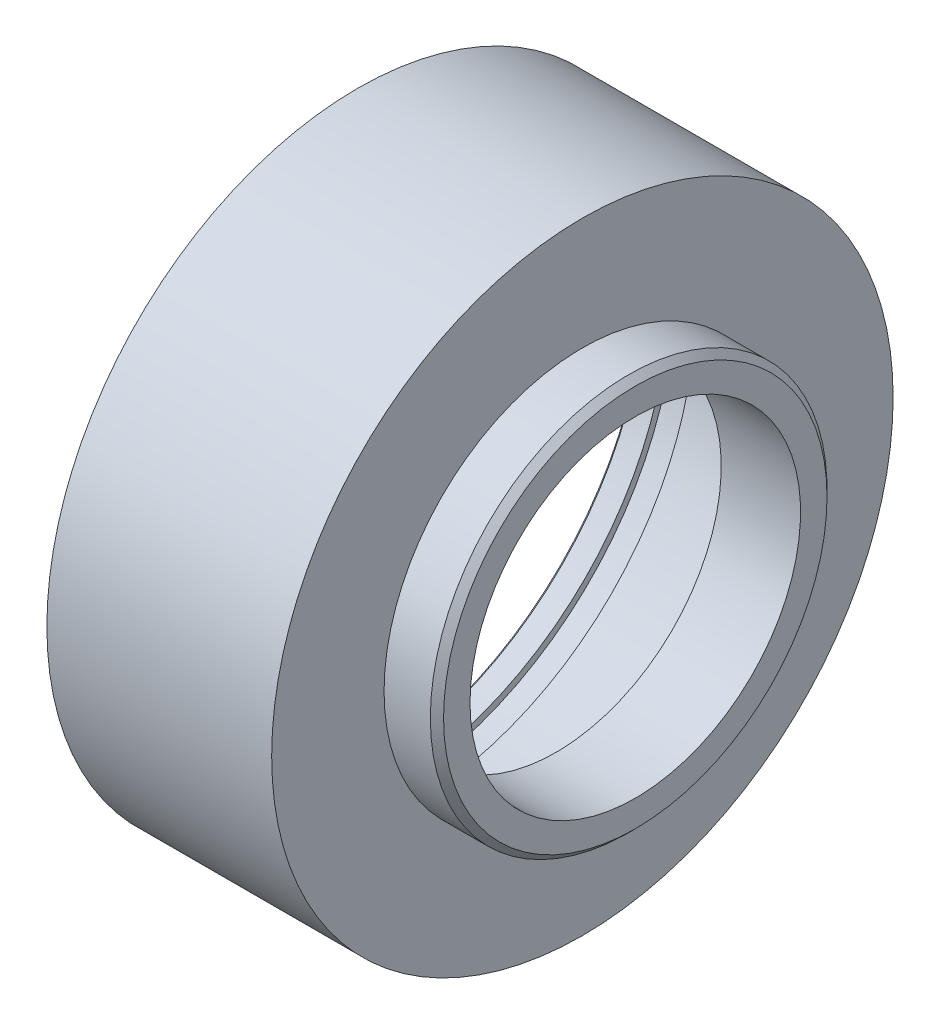
SolidWorks part; units mm, degrees
ref_plane "前视基准面" through (0, 0, 0) normal (0, 0, 1) x (1, 0, 0)
ref_plane "上视基准面" through (0, 0, 0) normal (0, 1, 0) x (1, 0, 0)
ref_plane "右视基准面" through (0, 0, 0) normal (1, 0, 0) x (0, 0, -1)
sketch "草图1" plane through (0, 0, 0) normal (0, 0, 1) x (1, 0, 0)
  line L0 (0, 0) -> (43.6676, 0) construction
  line L1 (2.1796, 21.5) -> (4.1796, 21.5)
  line L2 (4.1796, 22) -> (6.1796, 22)
  line L3 (6.1796, 22) -> (6.1796, 21.5)
  line L4 (6.1796, 21.5) -> (13.1796, 21.5)
  line L5 (13.1796, 21.5) -> (13.1796, 21)
  line L6 (13.1796, 21) -> (17.1796, 21)
  line L7 (17.1796, 21) -> (17.1796, 12.5)
  line L8 (17.1796, 12.5) -> (23.1796, 12.5)
  line L9 (23.1796, 12.5) -> (23.1796, 15)
  line L10 (23.1796, 15) -> (19.1796, 15)
  line L11 (2.1796, 23.5) -> (2.1796, 21.5)
  line L12 (4.1796, 22) -> (4.1796, 21.5)
  line L13 (19.1796, 15) -> (19.1796, 23.5)
  line L14 (19.1796, 23.5) -> (2.1796, 23.5)
  dimension "D1" = 21.5
  dimension "D2" = 43.6676
  dimension "D3" = 2
  dimension "D4" = 0.5
  dimension "D5" = 2
  dimension "D6" = 0.5
  dimension "D7" = 0.5
  dimension "D8" = 7
  dimension "D9" = 4
  dimension "D10" = 8.5
  dimension "D11" = 6
  dimension "D12" = 2.5
  dimension "D13" = 4
  dimension "D14" = 8.5
revolve "旋转1" add sketch "草图1" angle 360 about L0
chamfer "倒角1" distance 0.25 angle 45 1 edges at (2.1796, 0, 21.5)
chamfer "倒角2" distance 0.5 angle 45 1 edges at (23.1796, 0, 15)
